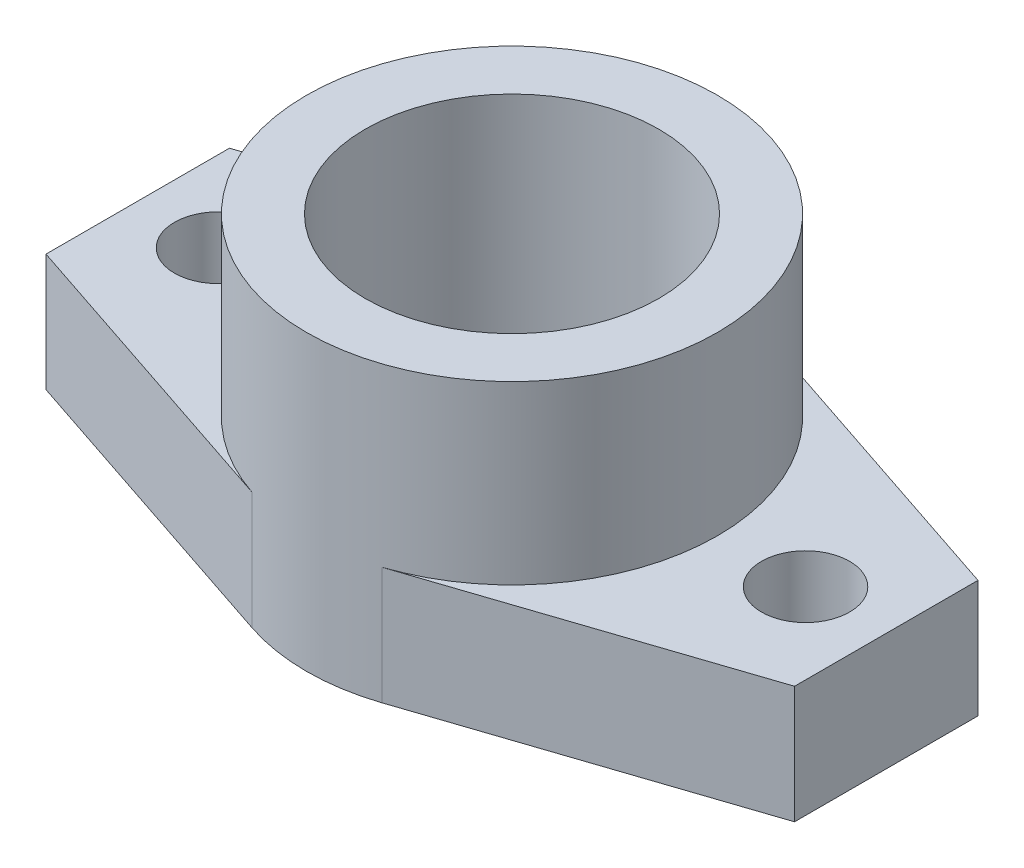
SolidWorks part; units mm, degrees
ref_plane "前视基准面" through (0, 0, 0) normal (0, 0, 1) x (1, 0, 0)
ref_plane "上视基准面" through (0, 0, 0) normal (0, 1, 0) x (1, 0, 0)
ref_plane "右视基准面" through (0, 0, 0) normal (1, 0, 0) x (0, 0, -1)
sketch "草图1" plane through (0, 0, 0) normal (0, 1, 0) x (1, 0, 0)
  circle A0 centre (0, 0) radius 28
  dimension "D1" = 56
extrude "凸台-拉伸1" add sketch "草图1" along normal blind 40
sketch "草图2" plane through (0, 0, 0) normal (0, -1, 0) x (1, 0, 0)
  line L0 (-51, -12.5) -> (-51, 12.5)
  line L1 (-51, 12.5) -> (-8.8627, 26.5604)
  line L2 (0, 0) -> (0, 46.0814) construction
  line L3 (0, 0) -> (-80.1367, 0) construction
  line L4 (-51, -12.5) -> (-8.8627, -26.5604)
  line L5 (-8.8627, 26.5604) -> (-8.8627, -26.5604)
  circle A0 centre (0, 0) radius 28 construction
  point P10 (-51, 0)
  dimension "D1" = 51
  dimension "D2" = 25
extrude "凸台-拉伸2" add sketch "草图2" against normal blind 16
mirror "镜向1" about plane through (0, 0, 0) normal (1, 0, 0) of "凸台-拉伸2"
sketch "草图3" plane through (0, 40, 0) normal (0, 1, 0) x (1, 0, 0)
  circle A0 centre (0, 0) radius 20
  dimension "D1" = 40
extrude "切除-拉伸1" cut sketch "草图3" against normal through all
sketch "草图4" plane through (0, 16, 0) normal (0, 1, 0) x (1, 0, 0)
  line L0 (0, 13.9095) -> (0, 0) construction
  line L1 (0, 0) -> (75.2994, 0) construction
  circle A0 centre (-40, 0) radius 6
  circle A1 centre (40, 0) radius 6
  dimension "D1" = 12
  dimension "D2" = 80
extrude "切除-拉伸2" cut sketch "草图4" against normal through all
